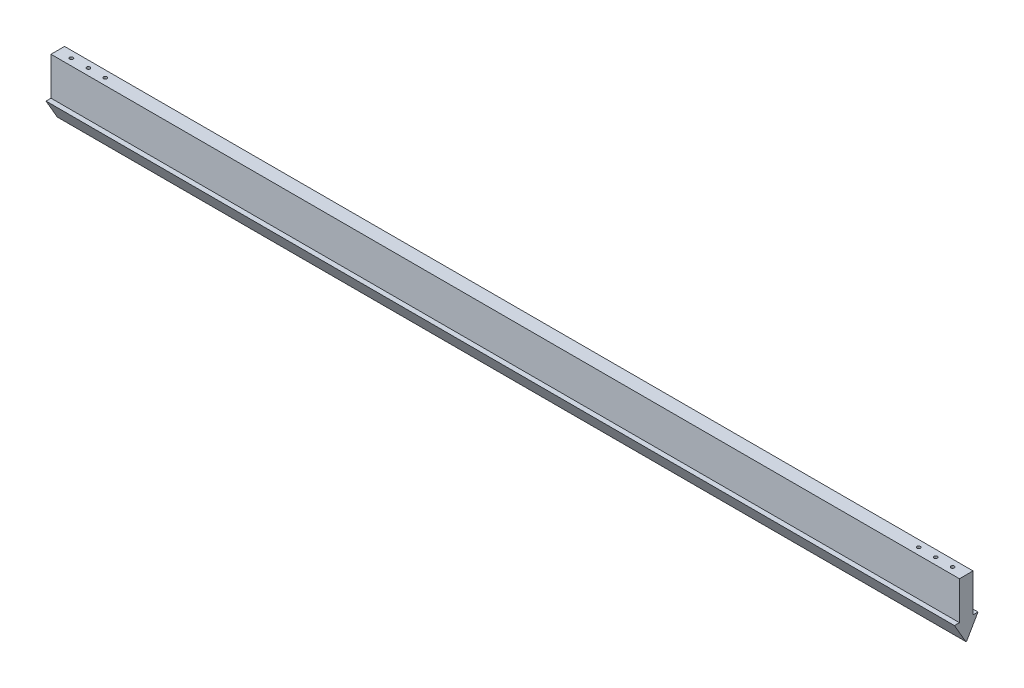
SolidWorks part; units mm, degrees
ref_plane "前视基准面" through (0, 0, 0) normal (0, 0, 1) x (1, 0, 0)
ref_plane "上视基准面" through (0, 0, 0) normal (0, 1, 0) x (1, 0, 0)
ref_plane "右视基准面" through (0, 0, 0) normal (1, 0, 0) x (0, 0, -1)
sketch "草图1" plane through (0, 0, 0) normal (1, 0, 0) x (0, 0, -1)
  line L0 (0, 0) -> (-17.3205, 30)
  line L1 (0, 0) -> (17.3205, 30)
  line L2 (0, 0) -> (0, 48.0317) construction
  line L3 (17.3205, 30) -> (10, 30)
  line L4 (10, 30) -> (10, 86)
  line L5 (10, 86) -> (-10, 86)
  line L6 (-10, 86) -> (-10, 30)
  line L7 (-10, 30) -> (-17.3205, 30)
  dimension "D1" = 60
  dimension "D2" = 30
  dimension "D3" = 20
  dimension "D4" = 56
extrude "凸台-拉伸1" add sketch "草图1" along normal blind 1337
fillet "圆角1" radius 1 1 edges at (668.5, 0, 0)
hole_wizard "M6 螺纹孔1" positions "草图2" profile "草图3" tap size "M6" standard "GB"
sketch "草图2" plane through (0, 86, 0) normal (0, 1, 0) x (1, 0, 0)
  line L0 (0, 0) -> (83.6552, 0) construction
  line L2 (0, 10) -> (0, -10) construction
  line L3 (1337, 10) -> (1337, -10) construction
  point P0 (20, 0)
  point P2 (45, 0)
  point P4 (70, 0)
  point P6 (1317, 0)
  point P8 (1292, 0)
  point P10 (1267, 0)
  dimension "D1" = 20
  dimension "D2" = 25
  dimension "D3" = 25
  dimension "D4" = 20
  dimension "D5" = 25
  dimension "D6" = 25
sketch "草图3" plane through (20, 86, 0) normal (1, 0, 0) x (0, 0, 1)
  line L0 (0, 0) -> (0, 16.5022)
  line L1 (0, 16.5022) -> (2.5, 15)
  line L2 (2.5, 15) -> (2.5, 0)
  line L5 (2.5, 0) -> (0, 0)
  line L10 (0, 16.5022) -> (-2.5, 15) construction
  line L11 (0, -6.35) -> (0, 107.95) construction
  dimension "螺纹孔钻头直径" = 5
  dimension "螺纹孔钻头深度" = 15
  dimension "导头角度" = 118
cosmetic thread "孔螺蚊线1" parameters "D1"=12, "D2"=6
cosmetic thread "孔螺蚊线2" parameters "D1"=12, "D2"=6
cosmetic thread "孔螺蚊线3" parameters "D1"=12, "D2"=6
cosmetic thread "孔螺蚊线4" parameters "D1"=12, "D2"=6
cosmetic thread "孔螺蚊线5" parameters "D1"=12, "D2"=6
cosmetic thread "孔螺蚊线6" parameters "D1"=12, "D2"=6
